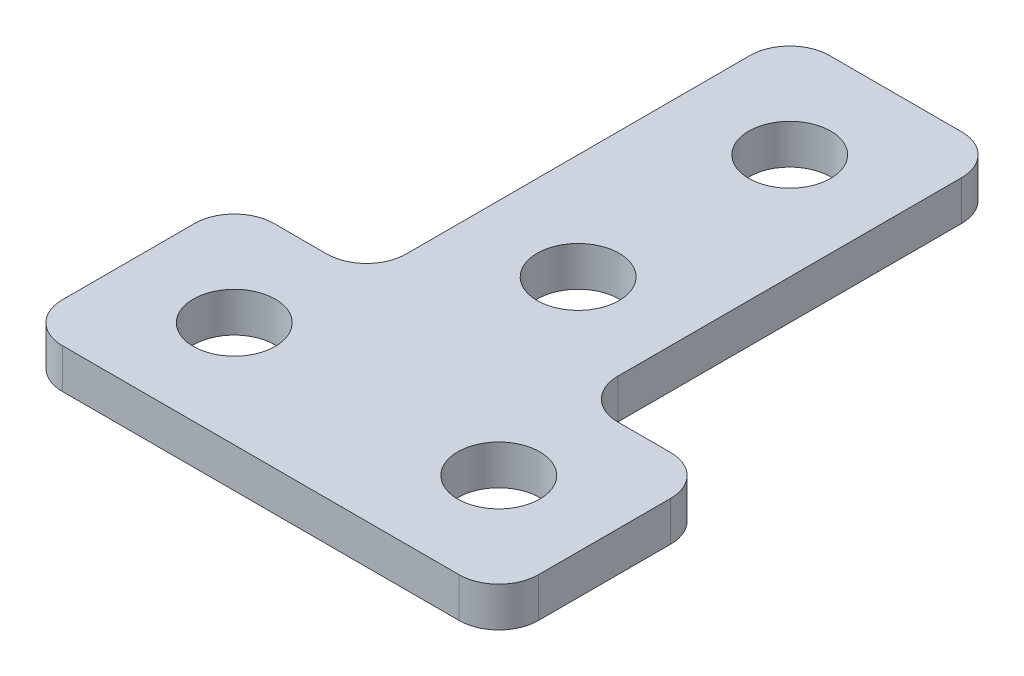
SolidWorks part; units mm, degrees
material "Thornel Mat VMA"
ref_plane "前视基准面" through (0, 0, 0) normal (0, 0, 1) x (1, 0, 0)
ref_plane "上视基准面" through (0, 0, 0) normal (0, 1, 0) x (1, 0, 0)
ref_plane "右视基准面" through (0, 0, 0) normal (1, 0, 0) x (0, 0, -1)
other "Configuration Table"
sketch "草图1" plane through (0, 0, 0) normal (0, 1, 0) x (1, 0, 0)
  line L0 (0, 0) -> (51.959, 0) construction
  line L1 (0, 0) -> (0, 49.2251) construction
  line L2 (-4, 20) -> (4, 20)
  line L3 (4, 20) -> (4, 4)
  line L4 (4, 4) -> (9, 4)
  line L5 (9, 4) -> (9, -4)
  line L6 (9, -4) -> (-9, -4)
  line L7 (-9, 4) -> (-9, -4)
  line L8 (-4, 4) -> (-9, 4)
  line L9 (-4, 20) -> (-4, 4)
  circle A0 centre (5, 0) radius 1.55
  circle A1 centre (0, 8) radius 1.55
  circle A2 centre (0, 16) radius 1.55
  circle A3 centre (-5, 0) radius 1.55
  point P12 (1.2355, -4.9949)
  point P20 (0, -4)
  point P23 (0, 20)
  dimension "D1" = 3.1
  dimension "D2" = 8
  dimension "D3" = 8
  dimension "D4" = 5
  dimension "D5" = 4
  dimension "D8" = 4
  dimension "D6" = 8
  dimension "D7" = 4
extrude "凸台-拉伸1" add sketch "草图1" along normal blind 1.5
fillet "圆角1" radius 1.5 8 edges at (4, 0.75, -4) (9, 0.75, -4) (9, 0.75, 4) (-4, 0.75, -4) (-4, 0.75, -20) (4, 0.75, -20) (-9, 0.75, 4) (-9, 0.75, -4)
